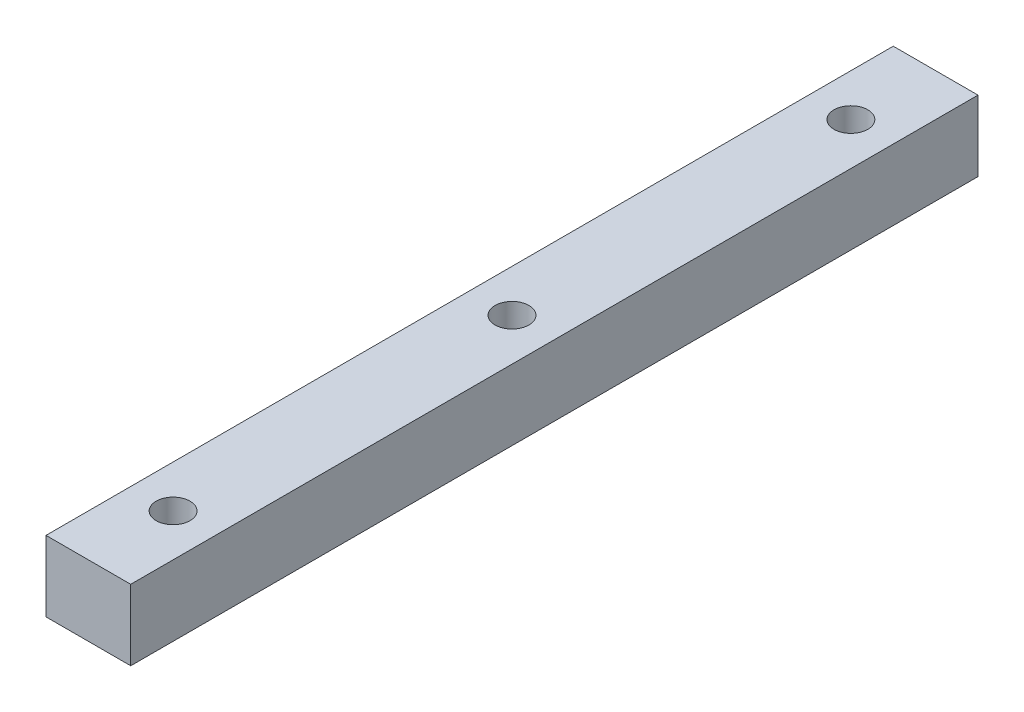
SolidWorks part; units mm, degrees
ref_plane "前视基准面" through (0, 0, 0) normal (0, 0, 1) x (1, 0, 0)
ref_plane "上视基准面" through (0, 0, 0) normal (0, 1, 0) x (1, 0, 0)
ref_plane "右视基准面" through (0, 0, 0) normal (1, 0, 0) x (0, 0, -1)
sketch "草图1" plane through (0, 0, 0) normal (0, 0, 1) x (1, 0, 0)
  line L1 (-7.5, 6.25) -> (7.5, 6.25)
  line L2 (-7.5, 6.25) -> (-7.5, -6.25)
  line L3 (-7.5, -6.25) -> (7.5, -6.25)
  line L4 (7.5, 6.25) -> (7.5, -6.25)
  line L5 (-7.5, 6.25) -> (7.5, -6.25) construction
  line L6 (-7.5, -6.25) -> (7.5, 6.25) construction
  point P0 (0, 0)
  dimension "D1" = 15
  dimension "D2" = 12.5
extrude "凸台-拉伸1" add sketch "草图1" along normal mid plane 150
sketch "草图2" plane through (0, 6.25, 0) normal (0, 1, 0) x (1, 0, 0)
  line L0 (0, -60) -> (0, -75) construction
  line L1 (7.5, -75) -> (-7.5, -75) construction
  circle A0 centre (0, -60) radius 3
  dimension "D2" = 6
  dimension "D1" = 15
extrude "切除-拉伸1" cut sketch "草图2" against normal blind 4.5
sketch "草图3" plane through (0, 6.25, 0) normal (0, 1, 0) x (1, 0, 0)
  circle A0 centre (0, -60) radius 2
  dimension "D1" = 4
extrude "切除-拉伸2" cut sketch "草图3" against normal through all
pattern_linear "阵列(线性)1" count 6 spacing 60 along (0, 0, -1) of "切除-拉伸1", "切除-拉伸2"
sketch "草图4" plane through (0, 6.25, 0) normal (0, 1, 0) x (1, 0, 0)
  line L1 (-155.28, 163.6462) -> (34.052, 163.6462)
  line L2 (-155.28, 163.6462) -> (-155.28, 30)
  line L3 (-155.28, 30) -> (34.052, 30)
  line L4 (34.052, 163.6462) -> (34.052, 30)
  line L5 (-155.28, 163.6462) -> (34.052, 30) construction
  line L6 (-155.28, 30) -> (34.052, 163.6462) construction
  point P0 (-60.614, 96.8231)
  dimension "D1" = 30
extrude "切除-拉伸3" [suppressed] cut sketch "草图4" against normal through all
